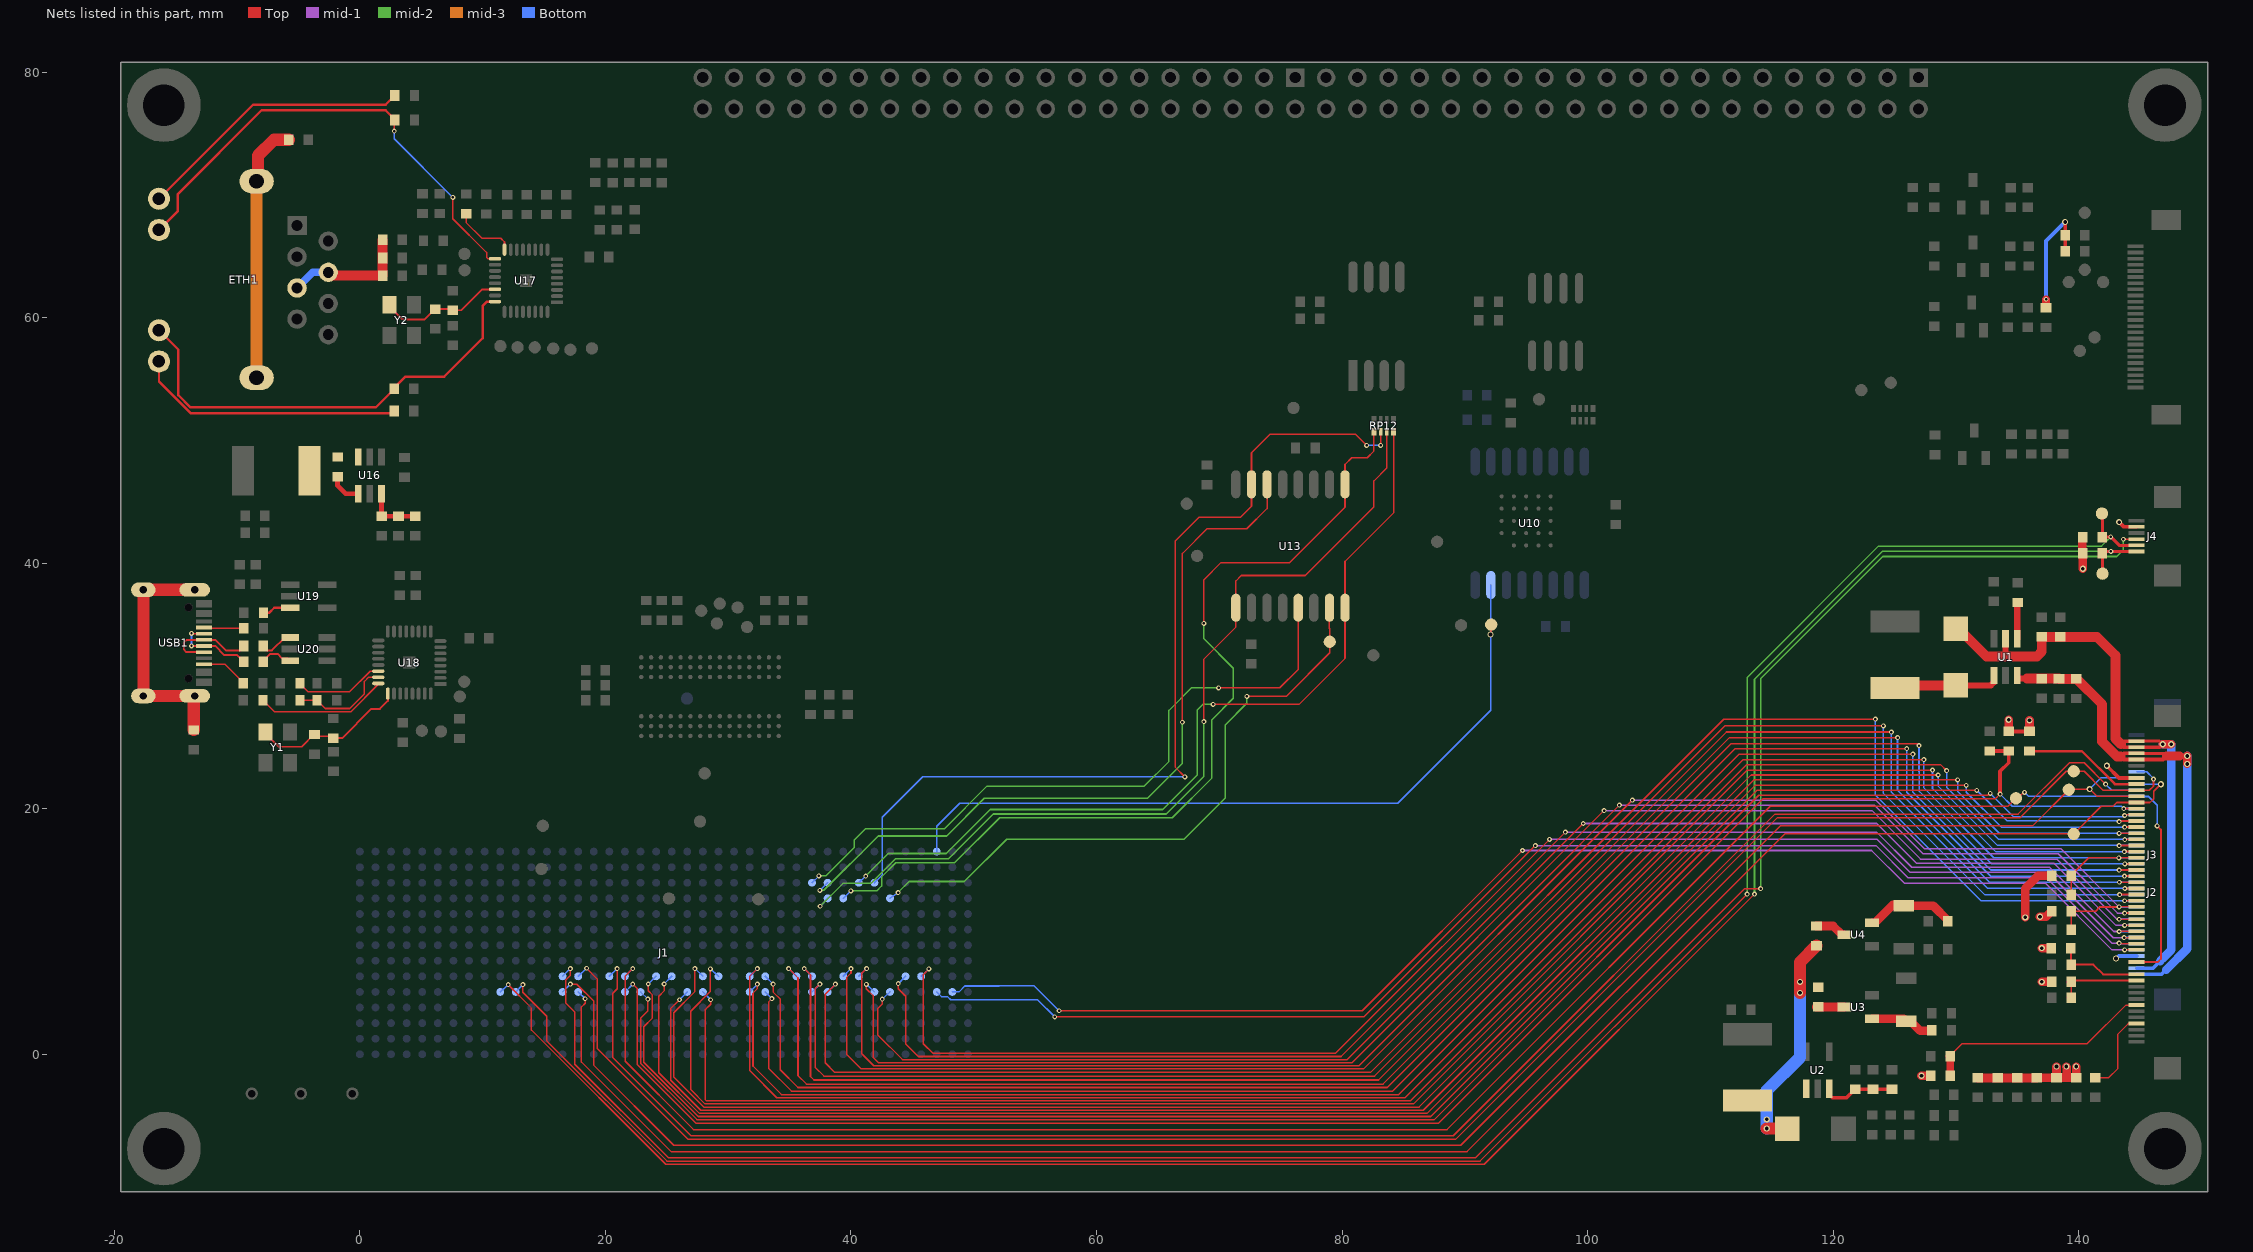
[diagram p0: the nets of this part, all layers, seen from the top]
# Altium PCB MISC105414.PcbDoc (part 7 of 11)
Units mm, origin at the board's own origin, x right, y up, seen from the top; angles counter-clockwise.
Board outline 170 x 92 mm, 6 copper layers (Top, GND, mid-1, mid-2, mid-3, Bottom), stack 1.231 mm thick; 238 components, 304 nets, 1456 pads, 1258 vias.
Unrouted connection lines stored in the file: 57.

## Via types
v1: diameter 0.4, hole 0.2, Top to Bottom, tented top, 618 vias
v2: diameter 0.5, hole 0.3, Top to Bottom, tented top, 522 vias
v3: diameter 0.5, hole 0.3, Top to Bottom, 41 vias
v4: diameter 1, hole 0.5, Top to Bottom, tented top, 36 vias
v5: diameter 0.7, hole 0.4, Top to Bottom, tented top, 34 vias
v6: diameter 1.3, hole 1.3, Top to Bottom, tented top, 3 vias
v7: diameter 4, hole 4, Top to Bottom, tented top, 2 vias
v8: diameter 3.3, hole 3.3, Top to Bottom, tented top, 2 vias

## Nets (pads, with @x,y where several pads share a name; then routed paths per layer and width w, separated by ;. In a path a pad name is that pad's centre, name@x,y a point inside that pad or via, vN(x,y) a via of type N, cw(c..) or ccw(c..) an arc to the next point about the centre after c; other vN are vias at no path point) (continued)
LCD_B0: J1.D17 J2.19 J3.21 | length 145.6
  Top w0.127: v1(28.544,6.958) 28.544,5.107 26.941,3.504 26.941,-2.865 28.119,-4.042 85.825,-4.042 113.017,23.15 v1(128.1,23.15)
  Top w0.15: v1(143.734,16.511) J2.19@144.73,16.51
  Bottom w0.127: v1(28.544,6.958) J1.D17@29.21,6.35 ; v1(128.1,23.15) 128.1,21.65 133.24,16.51 J3.21@144.73,16.51
LCD_B1: J1.D18 J2.18 J3.22 | length 146.2
  Top w0.127: v1(27.287,6.98) 27.287,5.107 25.567,3.387 25.567,-1.85 28.014,-4.296 86.275,-4.296 113.321,22.75 v1(128.55,22.75)
  Top w0.15: v1(143.297,16.994) 143.297,17.01 J2.18@144.73,17.01
  Bottom w0.127: v1(27.287,6.98) J1.D18@27.94,6.35 ; v1(128.55,22.75) 128.55,21.85 133.39,17.01 J3.22@144.73,17.01
LCD_B2: J1.C18 J2.17 J3.23 | length 141.5
  Top w0.127: v1(28.575,4.445) 28.575,4.082 28.12,3.626 28.12,-3.684 28.224,-3.788 85.575,-3.788 112.963,23.6 128.75,23.6 v1(129.25,23.1)
  Top w0.15: v1(143.76,17.486) 143.76,17.51 J2.17@144.73,17.51
  Bottom w0.127: J1.C18@27.94,5.08 v1(28.575,4.445) ; v1(129.25,23.1) 129.25,21.741 133.481,17.51 J3.23@144.73,17.51
LCD_B3: J1.C19 J2.16 J3.24 | length 143.1
  Top w0.127: v1(26.035,4.445) 25.313,3.723 25.313,-2.107 27.765,-4.56 86.625,-4.56 113.535,22.35 v1(130.15,22.35)
  Top w0.15: v1(143.3,18) 143.3,18.01 J2.16@144.73,18.01
  Bottom w0.127: v1(26.035,4.445) J1.C19@26.67,5.08 ; v1(130.15,22.35) 130.15,21.4 133.54,18.01 J3.24@144.73,18.01
LCD_B4: J1.D20 J2.15 J3.25 | length 143.8
  Top w0.127: v1(24.779,5.725) 24.779,5.162 24.345,4.728 24.345,-1.499 27.66,-4.814 86.925,-4.814 113.639,21.9 v1(130.85,21.9)
  Top w0.15: v1(143.75,18.5) 143.75,18.51 J2.15@144.73,18.51
  Bottom w0.127: v1(24.779,5.725) J1.D20@25.4,6.35 ; v1(130.85,21.9) 130.85,21.35 133.69,18.51 J3.25@144.73,18.51
LCD_B5: J1.D21 J2.14 J3.26 | length 144.6
  Top w0.127: v1(23.489,5.724) 23.489,5.172 23.827,4.834 23.827,2.947 23.132,2.252 23.132,-0.644 27.555,-5.068 87.225,-5.068 113.793,21.5 v1(131.7,21.5)
  Top w0.15: v1(143.3,18.95) 143.3,19.01 J2.14@144.73,19.01
  Bottom w0.127: v1(23.489,5.724) J1.D21@24.13,6.35 ; v1(131.7,21.5) 134.19,19.01 J3.26@144.73,19.01
LCD_B6: J1.C22 J2.13 J3.27 | length 143
  Top w0.127: v1(23.463,4.495) 23.463,3.537 22.877,2.951 22.877,-0.749 27.45,-5.322 87.525,-5.322 113.947,21.1 132.6,21.1 132.75,21.25 v1(132.8,21.25)
  Top w0.15: v1(143.75,19.45) 143.75,19.51 J2.13@144.73,19.51
  Bottom w0.127: J1.C22@22.86,5.08 v1(23.463,4.495) ; v1(132.8,21.25) 134.7,19.35 143.656,19.35 143.816,19.51 J3.27@144.73,19.51
LCD_B7: J1.C23 J2.12 J3.28 R6.1 R7.2 | length 149.7
  Top w0.127: v1(22.225,5.715) 22.589,5.351 22.589,-0.829 27.385,-5.625 87.849,-5.625 114.274,20.8 133.2,20.8 v1(133.6,21.2)
  Top w0.15: v1(143.679,20.013) 143.679,20.01 J2.12@144.73,20.01
  Top w0.3: R7.2@132.75,24.7 R6.1@134.3,24.7 134.3,23.748 133.6,23.048 v1(133.6,21.2)
  Bottom w0.127: J1.C23@21.59,5.08 v1(22.225,5.715) ; v1(133.6,21.2) 134.6,20.2 143.492,20.2 v1(143.679,20.013)
  Bottom w0.15: v1(143.679,20.013) 143.679,20.01 J3.28@144.73,20.01
LCD_BL_EN: R5.2 U1.4 | length 3
  Top w0.5: U1.4@135,33.85 135,36.75 R5.2@135.05,36.8
LCD_CLK: J1.D23 J2.37 J3.30 TP7.1 | length 162.3
  Top w0.127: v1(22.225,6.985) 21.607,6.367 21.607,-0.566 27.174,-6.133 88.549,-6.133 114.882,20.2 134.25,20.2 TP7.1@134.9,20.85
  Top w0.15: TP7.1@134.9,20.85 v1(135.594,21.337) ; J2.37@144.73,7.51 146.45,7.51 146.7,7.76 146.7,18.3 v1(146.4,18.6)
  Bottom w0.127: J1.D23@21.59,6.35 v1(22.225,6.985) ; v1(135.594,21.337) 135.921,21.01 J3.30@144.73,21.01
  Bottom w0.15: J3.30@144.73,21.01 145.69,21.01 146.4,20.3 v1(146.4,18.6)
LCD_DE: J1.D26 J2.9 J3.34 TP4.1 | length 153.1
  Top w0.127: v1(18.461,7.009) 19.321,6.149 19.321,0.485 26.715,-6.909 89.279,-6.909 115.438,19.25 135.2,19.25 139,23.05 TP4.1@139.6,23.05 140.45,23.05 141.99,21.51 J2.9@144.73,21.51
  Top w0.15: J2.9@144.73,21.51 145.76,21.51 146.1,21.85 v1(146.1,22.41)
  Bottom w0.127: J1.D26@17.78,6.35 v1(18.461,7.009)
  Bottom w0.15: J3.34@144.73,23.01 145.555,23.01 146.1,22.465 v1(146.1,22.41)
LCD_DISP: J1.D24 J3.31 | length 148.6
  Top w0.127: v1(20.955,6.985) 20.955,5.337 20.591,4.973 20.591,-0.268 26.964,-6.641 89.052,-6.641 115.26,19.567 135.067,19.567 139.25,23.75 140.45,23.75 v1(142.2,22)
  Bottom w0.127: J1.D24@20.32,6.35 v1(20.955,6.985) ; v1(142.2,22) 142.69,21.51 J3.31@144.73,21.51
LCD_DITHB: J2.47 R16.2 | length 6.8
  Top w0.127: R16.2@141.35,-1.9 142.45,-1.9 143.2,-1.15 143.2,1.65 144.06,2.51 J2.47@144.73,2.51
LCD_DVDD: C3.1 C4.1 C5.2 C6.2 J2.7 J3.4 J4.2 LR1.1 LR2.1 R1.2 R3.2 R6.2 R8.2 R10.2 R13.2 R15.2 R17.2 R18.2 | length 32
  Top w0.3: R6.2@134.3,26.3 R15.2@136,26.3 ; R1.2@137.55,11.4 R1.2@137.8,11.65 ; v2(142.3,23.5) 143.29,22.51 J2.7@144.73,22.51 ; v2(143.3,43.35) 143.69,42.96 J4.2@144.733,42.96
  Top w0.7: v2(127.2,-1.75) R13.2@127.95,-1.75 ; LR1.1@131.8,-1.9 131.8,-1.931 LR2.1@133.4,-1.931 ; LR2.1@133.4,-1.9 LR2.1@133.4,-1.931 ; R6.2@134.3,26.3 v2(134.3,27.25) ; C3.1@135,-1.9 C3.1@135,-1.931 ; v2(135.65,11.15) 135.65,13.5 136.7,14.55 R3.2@137.8,14.55 ; R15.2@136,26.3 v2(136,27.2) ; v2(136.85,11.2) 137.35,11.2 R1.2@137.8,11.65 ; v2(137,5.9) R10.2@137.8,5.9 ; v2(137,8.65) 137,8.625 R8.2@137.768,8.625 ; v2(138.2,-1) C5.2@138.2,-1.9 ; C5.2@138.2,-1.869 C5.2@138.2,-1.889 ; v2(139,-1) 139.05,-1.05 139.05,-1.889 ; C6.2@139.8,-1.9 C6.2@139.8,-1.889 ; v2(139.8,-1) C6.2@139.8,-1.87 ; R17.2@140.33,42.11 140.299,42.11 140.299,40.81 R18.2@140.33,40.81 140.33,39.55 v2(140.35,39.55) ; LR2.1@133.4,-1.931 C3.1@135,-1.931 ; C3.1@135,-1.931 136.6,-1.931 C4.1@136.6,-1.9 C5.2@138.2,-1.9 ; C5.2@138.2,-1.9 C5.2@138.2,-1.889 ; C5.2@138.2,-1.889 139.05,-1.889 ; 139.05,-1.889 C6.2@139.8,-1.889 ; C6.2@139.8,-1.889 C6.2@139.8,-1.87 ; C6.2@139.8,-1.889 C6.2@139.8,-1.87
  Bottom w0.3: v2(143.05,7.8) 143.26,8.01 J3.4@144.73,8.01
LCD_G0: J1.C10 J2.27 J3.13 | length 137.5
  Top w0.127: v1(38.735,5.715) 37.902,4.882 37.902,-0.697 38.68,-1.475 82.325,-1.475 111.1,27.3 v1(123.45,27.3)
  Top w0.15: v1(143.755,12.51) J2.27@144.73,12.51
  Bottom w0.127: J1.C10@38.1,5.08 v1(38.735,5.715) ; v1(123.45,27.3) 123.45,21.1 132.04,12.51 J3.13@144.73,12.51
LCD_G1: J1.C11 J2.26 J3.14 | length 137.9
  Top w0.127: v1(37.465,5.715) 37.102,5.352 37.102,-1.078 37.798,-1.775 82.654,-1.775 111.179,26.75 v1(124.1,26.75)
  Top w0.15: v1(143.341,13.012) 143.341,13.01 J2.26@144.73,13.01
  Bottom w0.127: J1.C11@36.83,5.08 v1(37.465,5.715) ; v1(124.1,26.75) 124.1,21.25 132.34,13.01 J3.14@144.73,13.01
LCD_G2: J1.D11 J2.25 J3.15 | length 138.9
  Top w0.127: v1(36.195,6.985) 36.703,6.477 36.703,-1.813 36.982,-2.092 82.975,-2.092 111.317,26.25 v1(124.75,26.25)
  Top w0.15: v1(143.762,13.504) 143.762,13.51 J2.25@144.73,13.51
  Bottom w0.127: v1(36.195,6.985) J1.D11@36.83,6.35 ; v1(124.75,26.25) 124.75,21.35 132.59,13.51 J3.15@144.73,13.51
LCD_G3: J1.D12 J2.24 J3.16 | length 139.8
  Top w0.127: v1(34.925,6.985) 35.687,6.223 35.687,-1.74 36.376,-2.429 83.342,-2.429 111.571,25.8 v1(125.25,25.8)
  Top w0.15: v1(143.32,14.014) 143.32,14.01 J2.24@144.73,14.01
  Bottom w0.127: v1(34.925,6.985) J1.D12@35.56,6.35 ; v1(125.25,25.8) 125.25,21.5 132.74,14.01 J3.16@144.73,14.01
LCD_G4: J1.C14 J2.23 J3.17 | length 137.7
  Top w0.127: v1(33.564,4.534) 33.292,4.262 33.292,-1.141 35.15,-2.999 84.125,-2.999 112.024,24.9 v1(126,24.9)
  Top w0.15: v1(143.738,14.512) 143.738,14.51 J2.23@144.73,14.51
  Bottom w0.127: J1.C14@33.02,5.08 v1(33.564,4.534) ; v1(126,24.9) 126,21.35 132.84,14.51 J3.17@144.73,14.51
LCD_G5: J1.C15 J2.22 J3.18 | length 140
  Top w0.127: v1(32.385,5.715) 32.385,5.352 32.022,4.988 32.022,-0.963 34.339,-3.28 84.625,-3.28 112.355,24.45 v1(126.5,24.45)
  Top w0.15: v1(143.305,15.004) 143.305,15.01 J2.22@144.73,15.01
  Bottom w0.127: J1.C15@31.75,5.08 v1(32.385,5.715) ; v1(126.5,24.45) 126.5,21.35 132.84,15.01 J3.18@144.73,15.01
LCD_G6: J1.D14 J2.21 J3.19 | length 138
  Top w0.127: v1(33.655,5.715) 33.655,5.08 34.237,4.498 34.237,-1.254 35.687,-2.704 83.684,-2.704 111.688,25.3 126.85,25.3 v1(127,25.15)
  Top w0.15: v1(143.767,15.516) 143.767,15.51 J2.21@144.73,15.51
  Bottom w0.127: J1.D14@33.02,6.35 v1(33.655,5.715) ; v1(127,25.15) 127,23.03 127.036,22.993 127.036,21.4 132.926,15.51 J3.19@144.73,15.51
LCD_G7: J1.D15 J2.20 J3.20 R3.1 R4.2 | length 146.9
  Top w0.127: v1(32.385,6.985) 31.768,6.368 31.768,-1.336 33.966,-3.534 85.125,-3.534 112.659,24 v1(127.4,24)
  Top w0.15: R4.2@139.4,13 R3.1@139.4,14.55 139.4,14.601 140.809,16.01 J2.20@144.73,16.01
  Bottom w0.127: J1.D15@31.75,6.35 v1(32.385,6.985) ; v1(127.4,24) 127.4,21.7 133.09,16.01 J3.20@144.73,16.01
  other v1: 143.286,16.003
LCD_HSYNC: J1.C26 J2.11 J3.32 TP6.1 | length 152.5
  Top w0.127: v1(18.35,4.525) 18.35,4.162 18.048,3.859 18.048,-0.63 25.347,-7.928 90.179,-7.928 116.057,17.95 TP6.1@139.6,17.95 141.85,20.2 142.8,20.2 143.11,20.51 J2.11@144.73,20.51 145.81,20.51 146.122,20.822 146.122,21.422 v2(146.7,22)
  Bottom w0.127: J1.C26@17.78,5.08 v1(18.35,4.525) ; J3.32@144.73,22.01 144.74,22 v2(146.7,22)
LCD_LED+: C9.1 C10.1 D1.2 J2.1 J2.2 J3.2 U1.5 | length 54.1
  Top w0.15: 138.007,34 C10.1@138.5,34
  Top w0.25: J2.1@144.73,25.51 146.59,25.51 v2(146.85,25.25)
  Top w0.3: J2.1@144.73,25.51 143.706,25.51 143.448,25.252 143.69,25.01 J2.2@144.73,25.01 146.598,25.01 v2(146.85,25.25)
  Top w0.5: 134,32.4 134.05,32.45 U1.5@134.05,33.85
  Top w0.7: v2(146.85,25.25) v2(147.55,25.25)
  Top w0.8: D1.2@130,34.65 130.25,34.65 132.5,32.4 134,32.4 136.6,32.4 137,32.8 C9.1@137,34 138.007,34 141.5,34 143,32.5 143,25.7 143.448,25.252
  Bottom w0.3: J3.2@144.73,7.01 146.06,7.01 146.64,7.59
  Bottom w0.7: 146.64,7.59 146.9,7.85 147.55,8.5 v2(147.55,25.25) v2(146.85,25.25)
LCD_LED-: C7.2 J2.3 J2.4 J3.1 R12.2 R14.2 U1.3 | length 44.2
  Top w0.25: J2.3@144.73,24.51 146.91,24.51 147.12,24.3 147.16,24.3 ; 148.25,24.228 148.25,24.3 ; v2@148.828,23.65 v2(148.85,23.65)
  Top w0.3: J2.3@144.73,24.51 143.679,24.51 143.421,24.253 143.664,24.01 J2.4@144.73,24.01 146.87,24.01 147.16,24.3 ; 148.25,24.3 v2(148.85,24.3)
  Top w0.5: U1.3@135,30.85 135,30.6 135.725,30.6 135.8,30.675 135.8,30.6
  Top w0.7: 147.16,24.3 148.25,24.3 ; v2(148.85,23.65) v2(148.85,24.3)
  Top w0.8: 135.8,30.6 C7.2@137,30.6 138.4,30.6 R14.2@138.4,30.582 139.851,30.582 141.914,28.519 141.914,25.475 143.137,24.253 143.421,24.253
  Bottom w0.3: J3.1@144.73,6.51 146.76,6.51 147.15,6.9
  Bottom w0.7: 147.15,6.9 148.85,8.6 v2(148.85,23.65) v2(148.85,24.3)
LCD_LR: J2.39 R8.1 R9.2 | length 7
  Top w0.15: R8.1@139.368,8.625 139.392,8.625 R9.2@139.392,7.3 141.2,7.3 141.99,6.51 J2.39@144.73,6.51
LCD_MODE: J2.8 R15.1 | length 9.8
  Top w0.2: R15.1@136,24.7 140.26,24.7 142.95,22.01 J2.8@144.73,22.01
LCD_R0: J1.C2 J2.35 J3.5 | length 107.3
  Top w0.127: v1(56.95,3.55) 81.65,3.55 v1(94.7,16.6) ; v1(143.75,8.5) 143.75,8.51 J2.35@144.73,8.51
  mid-1 w0.127: v1(94.7,16.6) 123.135,16.6 125.811,13.924 137.295,13.924 142.719,8.5 v1(143.75,8.5)
  Bottom w0.127: J1.C2@48.26,5.08 48.795,5.08 49.278,5.564 52.071,5.564 52.107,5.6 54.9,5.6 v1(56.95,3.55)
  Bottom w0.15: v1(143.75,8.5) 143.75,8.51 J3.5@144.73,8.51
LCD_R1: J1.C3 J2.34 J3.6 | length 109.2
  Top w0.127: v1(56.6,3.05) 81.8,3.05 v1(95.75,17) ; v1(143.3,9.05) 143.3,9.01 J2.34@144.73,9.01
  mid-1 w0.127: v1(95.75,17) 123.488,17 126.108,14.38 137.388,14.38 142.717,9.05 v1(143.3,9.05)
  Bottom w0.127: J1.C3@46.99,5.08 47.369,4.701 47.867,4.701 48.123,4.445 55.205,4.445 v1(56.6,3.05)
  Bottom w0.15: v1(143.3,9.05) 143.3,9.01 J3.6@144.73,9.01
LCD_R2: J1.D4 J2.33 J3.7 | length 117.9
  Top w0.127: v1(46.35,6.95) 45.886,6.486 45.886,0.867 46.678,0.075 79.475,0.075 v1(96.9,17.5) ; v1(143.7,9.5) 143.7,9.51 J2.33@144.73,9.51
  mid-1 w0.127: v1(96.9,17.5) 123.591,17.5 126.262,14.829 137.492,14.829 142.821,9.5 v1(143.7,9.5)
  Bottom w0.127: J1.D4@45.72,6.35 v1(46.35,6.95)
  Bottom w0.15: v1(143.7,9.5) 143.7,9.51 J3.7@144.73,9.51
LCD_R3: J1.D5 J2.32 J3.8 | length 119.1
  Top w0.127: v1(43.85,5.75) 43.85,5.345 44.468,4.728 44.468,0.833 45.479,-0.179 79.921,-0.179 v1(98.2,18.1) ; v1(143.3,10) 143.3,10.01 J2.32@144.73,10.01
  mid-1 w0.127: v1(98.2,18.1) 123.542,18.1 126.416,15.226 137.639,15.226 142.865,10 v1(143.3,10)
  Bottom w0.127: v1(43.85,5.75) J1.D5@44.45,6.35
  Bottom w0.15: v1(143.3,10) 143.3,10.01 J3.8@144.73,10.01
LCD_R4: J1.C6 J2.31 J3.9 | length 119.7
  Top w0.127: v1(42.55,4.5) 42.55,4.097 42.182,3.729 42.182,1.575 44.19,-0.433 80.417,-0.433 v1(99.65,18.8) ; v1(143.75,10.5) 143.75,10.51 J2.31@144.73,10.51
  mid-1 w0.127: v1(99.65,18.8) 123.55,18.8 126.794,15.556 137.995,15.556 143.051,10.5 v1(143.75,10.5)
  Bottom w0.127: v1(42.55,4.5) J1.C6@43.18,5.08
  Bottom w0.15: v1(143.75,10.5) 143.75,10.51 J3.9@144.73,10.51
LCD_R5: J1.C7 J2.30 J3.10 | length 123.8
  Top w0.127: v1(41.25,5.7) 41.25,5.345 41.799,4.797 41.799,-0.249 42.237,-0.687 80.813,-0.687 v1(101.35,19.85) ; v1(143.3,11) 143.3,11.01 J2.30@144.73,11.01
  mid-1 w0.127: v1(101.35,19.85) 123.164,19.85 127.113,15.901 138.219,15.901 143.121,11 v1(143.3,11)
  Bottom w0.127: v1(41.25,5.7) J1.C7@41.91,5.08
  Bottom w0.15: v1(143.3,11) 143.3,11.01 J3.10@144.73,11.01
LCD_R6: J1.D8 J2.29 J3.11 | length 125.7
  Top w0.127: v1(41.275,6.985) 40.886,6.596 40.886,0.039 41.866,-0.941 81.376,-0.941 99.425,17.108 99.425,17.125 v1(102.6,20.3) ; v1(143.75,11.5) 143.75,11.51 J2.29@144.73,11.51
  mid-1 w0.127: v1(102.6,20.3) 123.36,20.3 127.335,16.325 138.342,16.325 143.167,11.5 v1(143.75,11.5)
  Bottom w0.127: J1.D8@40.64,6.35 v1(41.275,6.985)
  Bottom w0.15: v1(143.75,11.5) 143.75,11.51 J3.11@144.73,11.51
LCD_R7: J1.D9 J2.28 J3.12 R1.1 R2.2 | length 133.3
  Top w0.127: v1(40.005,6.985) 40.005,6.622 39.642,6.258 39.642,0.009 40.845,-1.195 81.755,-1.195 v1(103.65,20.7) ; v1(143.3,12) 143.3,12.01 J2.28@144.73,12.01
  Top w0.15: R2.2@139.4,10.15 R1.1@139.4,11.65 141.381,11.65 141.731,12 v1(143.3,12)
  mid-1 w0.127: v1(103.65,20.7) 123.497,20.7 127.455,16.742 138.558,16.742 v1(143.3,12)
  Bottom w0.127: J1.D9@39.37,6.35 v1(40.005,6.985)
  Bottom w0.15: v1(143.3,12) 143.3,12.01 J3.12@144.73,12.01
LCD_RSTN: C8.2 J2.44 R13.1 | length 18.6
  Top w0.125: C8.2@129.55,-0.15 129.55,-0.099 130.499,0.85 140.69,0.85 143.85,4.01 J2.44@144.73,4.01
  Top w0.6: C8.2@129.469,-0.15 C8.2@129.55,-0.15 R13.1@129.55,-1.75
LCD_TP_INT: J1.D27 J4.4 | length 170.9
  Top w0.127: v1(17.145,6.985) 17.145,6.425 16.782,6.062 16.782,4.164 17.503,3.443 17.503,-0.803 25.136,-8.436 90.879,-8.436 112.815,13.5 v1(114.1,13.5) ; v1(143.65,41.95) 143.65,41.96 J4.4@144.733,41.96
  mid-2 w0.127: v1(114.1,13.5) 114.1,30.6 124.05,40.55 143.1,40.55 143.65,41.1 v1(143.65,41.95)
  Bottom w0.127: J1.D27@16.51,6.35 v1(17.145,6.985)
LCD_TP_SCL: J1.C31 J4.6 R18.1 TP8.1 | length 174.1
  Top w0.127: v1(12.082,5.671) 13.974,3.779 13.974,1.976 24.905,-8.955 91.595,-8.955 v1(113.6,13.05)
  Top w0.25: TP8.1@141.95,39.15 141.95,40.81 R18.1@141.93,40.81 141.93,40.959 v1(142.636,40.959) 143.459,40.959 143.46,40.96 J4.6@144.733,40.96
  mid-2 w0.127: v1(113.6,13.05) 113.6,30.55 124.009,40.959 v1(142.636,40.959)
  Bottom w0.127: J1.C31@11.43,5.08 v1(12.082,5.671)
LCD_TP_SDA: J1.C30 J4.5 R17.1 TP9.1 | length 174.1
  Top w0.127: v1(13.274,5.674) 13.274,5.053 15.225,3.103 15.225,1.085 25.01,-8.701 91.249,-8.701 v1(113,13.05)
  Top w0.25: TP9.1@141.9,44.05 141.93,44.05 R17.1@141.93,42.15 ; R17.1@141.93,42.11 R17.1@141.93,42.15 ; J4.5@144.733,41.46 143.306,41.46 v1(142.616,42.15) R17.1@141.93,42.15
  mid-2 w0.127: v1(113,13.05) 113,30.7 123.7,41.4 141.865,41.4 v1(142.616,42.15)
  Bottom w0.127: J1.C30@12.7,5.08 v1(13.274,5.674)
LCD_UD: J2.40 R10.1 R11.2 | length 7.3
  Top w0.15: R11.2@139.094,4.6 R11.2@139.4,4.6 R10.1@139.4,5.9 ; R10.1@139.094,5.9 R10.1@139.4,5.9 ; J2.40@144.73,6.01 139.71,6.01 139.6,5.9 R10.1@139.4,5.9
LCD_VSYNC: J1.C27 J2.10 J3.33 TP5.1 | length 153.5
  Top w0.127: v1(17.145,5.715) 17.675,5.715 19.061,4.328 19.061,-0.903 25.575,-7.417 89.679,-7.417 115.696,18.6 136.25,18.6 TP5.1@139.2,21.55 139.25,21.6 v2(140.9,21.6) 141.49,21.01 J2.10@144.73,21.01
  Bottom w0.127: J1.C27@16.51,5.08 v1(17.145,5.715) ; v2(140.9,21.6) 141.81,22.51 J3.33@144.73,22.51
LED_LINK: ETH1.10 R47.2 U17.17 | length 39.5
  Top w0.127: v1(2.8,75.2) 2.8,76.103 R47.2@2.843,76.103 ; v1(7.573,69.798) 7.573,68.053 10.316,65.31 10.316,64.92 10.426,64.81 U17.17@11.002,64.81
  Top w0.2: ETH1.10@-16.365,67.145 -14.85,68.66 -14.85,70.05 -8,76.9 2.096,76.9 2.843,76.154 R47.2@2.843,76.103
  Bottom w0.127: v1(2.8,75.2) 2.8,74.571 v1(7.573,69.798)
LED_SPEED: ETH1.11 R48.2 U17.24 | length 37.4
  Top w0.2: ETH1.11@-16.365,58.975 -14.8,57.41 -14.8,53.7 -13.789,52.689 1.289,52.689 R48.2@2.8,54.2 2.775,54.2 2.775,54.275 3.7,55.2 6.875,55.2 10,58.325 10,60.96 10.35,61.31 U17.24@11.002,61.31
NETC12_1: C12.1 U3.3 | length 2.3
  Top w0.7: C12.1@118.65,3.85 118.806,3.85 120.7,3.85 U3.3@120.925,3.85
NETC12_2: C12.2 C13.2 D2.1 L2.2 U2.1 | length 19.1
  Top w1: v2(114.6,-6.05) D2.1@116.25,-6.05 ; v2(117.3,5) v2(117.3,5.9) 117.3,7.5 C13.2@118.65,8.85
  Bottom w1: v2(114.6,-6.05) v2(114.6,-5.3) 114.6,-2.95 117.3,-0.25 v2(117.3,5) v2(117.3,5.9)
NETC13_1: C13.1 U4.3 | length 2.6
  Top w0.7: C13.1@118.65,10.45 120,10.45 120.7,9.75 U4.3@120.925,9.75
NETC14_1: C14.1 R19.1 R20.2 U2.3 | length 6
  Top w0.3: U2.3@119.69,-2.797 119.69,-3.317 119.922,-3.55 121.1,-3.55 R20.2@121.8,-2.85 R19.1@123.25,-2.85 123.301,-2.85 124.749,-2.85 C14.1@124.8,-2.85
NETC15_1: C15.1 DZ2.1 U3.1 | length 5.3
  Top w0.7: U3.1@123.175,2.9 125.75,2.9 DZ2.1@125.95,2.7 126.3,2.7 127.093,1.907 128.05,1.907 C15.1@128.05,1.95
NETC16_1: C16.1 DZ1.2 U4.2 | length 7.4
  Top w0.7: U4.2@123.175,10.7 123.4,10.7 124.861,12.161 125.75,12.161 DZ1.2@125.75,12.1 128.151,12.1 129.35,10.901 C16.1@129.35,10.85
NETC76_1: C76.1 U16.1 | length 2.7
  Top w0.4: C76.1@-1.818,47.047 -1.818,46.318 -1.161,45.661 U16.1@-0.138,45.661
NETC76_2: C76.2 L3.1 U16.6
NETC81_2: C81.2 R30.2 R31.1 U16.3 | length 4.6
  Top w0.4: U16.3@1.762,45.661 1.771,45.652 R31.1@1.771,43.825 C81.2@3.146,43.825 R30.2@4.521,43.825
NETC83_1: C83.1 R32.1 U18.25 Y1.3 | length 13.1
  Top w0.15: Y1.3@-7.7,26.25 -7.7,26.125 -6.625,25.05 -4.751,25.05 -3.751,26.05 R32.1@-3.7,26.05 -3.7,25.9 -2.174,25.9 C83.1@-2.174,25.75 -1.45,25.75 0.928,28.128 1.628,28.128 2.28,28.78 U18.25@2.28,29.382
NETC86_1: C86.1 R33.1 U17.22 Y2.3 | length 10.3
  Top w0.15: Y2.3@2.4,61.05 2.4,60.925 3.475,59.85 5.249,59.85 6.099,60.7 7.55,60.7 C86.1@7.55,60.6 8.25,60.6 9.96,62.31 U17.22@11.002,62.31
NETC94_2: C94.2 C95.2 ETH1.4 ETH1.5 LR7.2 | length 10.5
  Top w0.8: ETH1.4@-2.575,63.695 -2.307,63.427 C94.2@1.852,63.427 1.852,63.478 1.853,64.812 1.853,64.913 1.852,66.289 LR7.2@1.852,66.34
  Bottom w0.6: ETH1.5@-5.115,62.425 -3.845,63.695 ETH1.4@-2.575,63.695
NETD1_1: D1.1 L1.2 U1.1 | length 8.9
  Top w0.5: D1.1@130,30.05 132.85,30.05 133.1,30.3 U1.1@133.1,30.85
  Top w0.8: L1.2@125.05,29.85 125.05,30.05 D1.1@130,30.05
NETETH1_9: ETH1.9 R52.2 | length 22.7
  Top w0.2: ETH1.9@-16.365,69.685 -8.7,77.35 2.09,77.35 R52.2@2.843,78.103
NETETH1_12: ETH1.12 R53.2 | length 22
  Top w0.2: ETH1.12@-16.365,56.435 -16.365,54.8 -13.766,52.201 2.601,52.201 R53.2@2.8,52.4
NETETH1_SH1: ETH1.SH1 ETH1.SH2 LR9.2 | length 21.2
  Top w1: ETH1.SH1@-8.415,71.105 -8.3,71.22 -8.3,73.2 -7,74.5 LR9.2@-5.8,74.5
  mid-3 w1: ETH1.SH2@-8.415,55.115 ETH1.SH1@-8.415,71.105
NETLR8_2: LR8.2 USB1.S1 USB1.S2 USB1.S3 USB1.S4 | length 19.8
  Top w1: LR8.2@-13.53,26.412 -13.53,29.144 USB1.S3@-13.484,29.19 ; USB1.S3@-13.453,29.19 USB1.S3@-13.484,29.19 ; USB1.S1@-13.453,37.83 USB1.S2@-17.632,37.83 USB1.S4@-17.632,29.19 USB1.S3@-13.484,29.19
NETR25_2: R25.2 R26.2 R27.2 | length 10
  Top w0.3: R26.2@138.9,65.4 R27.2@138.9,66.7 v2(138.9,67.8)
  Top w0.65: R25.2@137.343,60.803 137.343,61.5 v1(137.35,61.5)
  Bottom w0.3: v1(137.35,61.5) 137.35,66.25 v2(138.9,67.8)
NETR34_1: R34.1 U18.24 | length 10.8
  Top w0.127: R34.1@-7.892,28.836 -6.963,27.907 -0.725,27.907 1.502,30.134 U18.24@1.502,30.21
NETR35_1: R35.1 U18.22 | length 7.4
  Top w0.127: R35.1@-4.874,30.236 -4.874,30.185 -4.218,29.529 -0.843,29.529 0.838,31.21 U18.22@1.502,31.21
NETR36_1: R36.1 R37.1 U18.23 | length 8.3
  Top w0.127: R36.1@-4.874,28.836 R37.1@-3.492,28.836 -2.823,28.167 -0.825,28.167 0.367,29.359 0.367,30.368 0.709,30.71 U18.23@1.502,30.71
NETR39_2: R39.2 U17.16 | length 5.1
  Top w0.127: R39.2@8.652,68.473 8.652,67.759 9.937,66.475 11.48,66.475 11.78,66.175 U17.16@11.78,65.538
NETR46_2: R46.2 U19.3 | length 2.4
  Top w0.2: R46.2@-7.855,35.98 -7.374,35.98 -6.977,36.378 U19.3@-5.658,36.378
NETR49_1: R49.1 U20.4 | length 2.8
  Top w0.15: R49.1@-7.87,33.26 -7.87,33.209 -7.564,32.903 -7.486,32.903 -7.476,32.893 -7.162,32.893 -6.095,33.96 U20.4@-5.67,33.96
NETR49_2: R49.2 USB1.6 USB1.8 | length 7.8
  Top w0.15: USB1.8@-12.707,32.76 -14.13,32.76 -14.351,32.981 -14.351,33.528 -14.119,33.76 USB1.6@-12.707,33.76 -11.789,33.76 -10.922,32.893 -9.864,32.893 -9.854,32.903 -9.776,32.903 -9.47,33.209 R49.2@-9.47,33.26
NETR50_1: R50.1 U20.6 | length 2.7
  Top w0.15: R50.1@-7.87,31.985 -7.87,32.036 -7.29,32.616 -6.708,32.616 -6.352,32.26 -5.87,32.26 U20.6@-5.67,32.06
NETR50_2: R50.2 USB1.5 USB1.7 | length 6.8
  Top w0.15: v1(-13.716,33.274) -13.702,33.26 USB1.7@-12.707,33.26 -11.797,33.26 -11.049,32.512 -9.997,32.512 -9.827,32.342 -9.776,32.342 -9.47,32.036 R50.2@-9.47,31.985 ; v1(-13.716,34.29) -13.686,34.26 USB1.5@-12.707,34.26
  Bottom w0.15: v1(-13.716,33.274) v1(-13.716,34.29)
NETR51_2: R51.2 USB1.4 | length 3.3
  Top w0.15: USB1.4@-12.707,34.76 -12.653,34.705 R51.2@-9.455,34.705
NETR54_2: R54.2 USB1.10 | length 3.9
  Top w0.127: USB1.10@-12.707,31.76 -10.965,31.76 -9.492,30.286 R54.2@-9.492,30.236
NOR2_CS: J1.M3 TP21.1 U10.7 | length 63
  Top w0.127: v2(92.1,34.2) 92.15,34.25 TP21.1@92.15,35 v2(92.1,34.2)
  Bottom w0.127: J1.M3@46.99,16.51 46.99,18.582 48.858,20.45 84.55,20.45 92.125,28.025 v2@92.125,34.2 ; v2(92.1,34.2) 92.1,34.375 92.125,34.4 U10.7@92.125,38.225
NOR_CS: J1.J6 TP35.1 U13.7 | length 51.6
  Top w0.127: v1(72.25,29.15) 75.45,29.15 79,32.7 TP35.1@79,33.6 79,34.654 78.975,34.678 U13.7@78.975,36.375
  mid-2 w0.127: v1(43.838,13.169) 44.742,14.074 49.229,14.074 52.681,17.526 67.131,17.526 70.5,20.895 70.5,26.85 72.25,28.6 v1(72.25,29.15)
  Bottom w0.127: J1.J6@43.18,12.7 v1(43.838,13.169)
NOR_D0: J1.K7 RP12.2 U13.15 | length 75.5
  Top w0.127: v1(67.2,22.6) 66.4,23.4 66.4,41.8 68.35,43.75 71.725,43.75 72.625,44.65 72.625,49 74.125,50.5 81.1,50.5 v1(82,49.6) ; v1(83.15,49.6) RP12.2@83.15,50.7
  Bottom w0.127: J1.K7@41.91,13.97 41.91,13.978 42.545,14.613 42.545,19.3 45.845,22.6 v1(67.2,22.6) ; v1(82,49.6) v1(83.15,49.6)
NOR_D1: J1.K8 RP12.4 U13.8 | length 70.4
  Top w0.127: v1(69.5,28.5) 76.5,28.5 80.245,32.245 80.245,34.4 U13.8@80.245,36.375 80.245,40.145 84.2,44.1 RP12.4@84.2,50.7
  mid-2 w0.127: v1(41.206,14.519) 43.044,16.358 47.765,16.358 51.346,19.939 65.395,19.939 68.2,22.744 68.2,28.05 68.65,28.5 v1(69.5,28.5)
  Bottom w0.127: J1.K8@40.64,13.97 v1(41.206,14.519)
NOR_D2: J1.J9 RP12.1 U13.9 | length 74.2
  Top w0.127: v1(68.75,35.1) 68.75,38.65 70.15,40.05 75.745,40.05 80.245,44.55 U13.9@80.245,46.425 80.245,48.045 80.8,48.6 82.05,48.6 82.6,49.15 82.6,49.6 RP12.1@82.6,50.7
  mid-2 w0.127: v1(39.999,13.311) 42.1,13.311 42.498,13.709 42.498,14.437 43.656,15.595 48.44,15.595 52.119,19.274 66.174,19.274 69.4,22.5 69.4,27.25 71.15,29 71.15,31.45 68.75,33.85 v1(68.75,35.1)
  Bottom w0.127: J1.J9@39.37,12.7 39.981,13.311 v1(39.999,13.311)
NOR_D3: J1.J10 RP12.3 U13.1 | length 73.8
  Top w0.127: v1(68.75,27.1) 68.75,32.195 71.355,34.8 71.355,38.555 71.8,39 77,39 82.6,44.6 82.6,46.7 83.65,47.75 RP12.3@83.65,50.7
  mid-2 w0.127: v1(37.489,12.056) 39.347,13.915 41.631,13.915 41.938,14.222 41.938,14.236 43.629,15.927 47.943,15.927 51.59,19.574 65.684,19.574 68.75,22.64 v1(68.75,27.1)
  Bottom w0.127: v1(37.489,12.056) J1.J10@38.1,12.7
NOR_D4: J1.K10 U13.14 | length 62.2
  Top w0.127: v1(67,27.05) 67,40.8 69,42.8 72.245,42.8 73.895,44.45 U13.14@73.895,46.425
  mid-2 w0.127: v1(37.471,13.355) 37.791,13.355 42.216,17.78 47.8,17.78 50.867,20.847 64.147,20.847 67,23.7 v1(67,27.05)
  Bottom w0.127: v1(37.471,13.355) J1.K10@38.1,13.97
NOR_D5: J1.K11 U13.5 | length 54.6
  Top w0.127: v1(69.95,29.85) 74.935,29.85 76.435,31.35 U13.5@76.435,36.375
  mid-2 w0.127: v1(37.389,14.529) 37.955,14.529 40.271,16.845 40.271,17.45 41.192,18.371 47.612,18.371 51.088,21.847 63.897,21.847 65.9,23.85 65.9,28.003 67.747,29.85 v1(69.95,29.85)
  Bottom w0.127: J1.K11@36.83,13.97 v1(37.389,14.529)